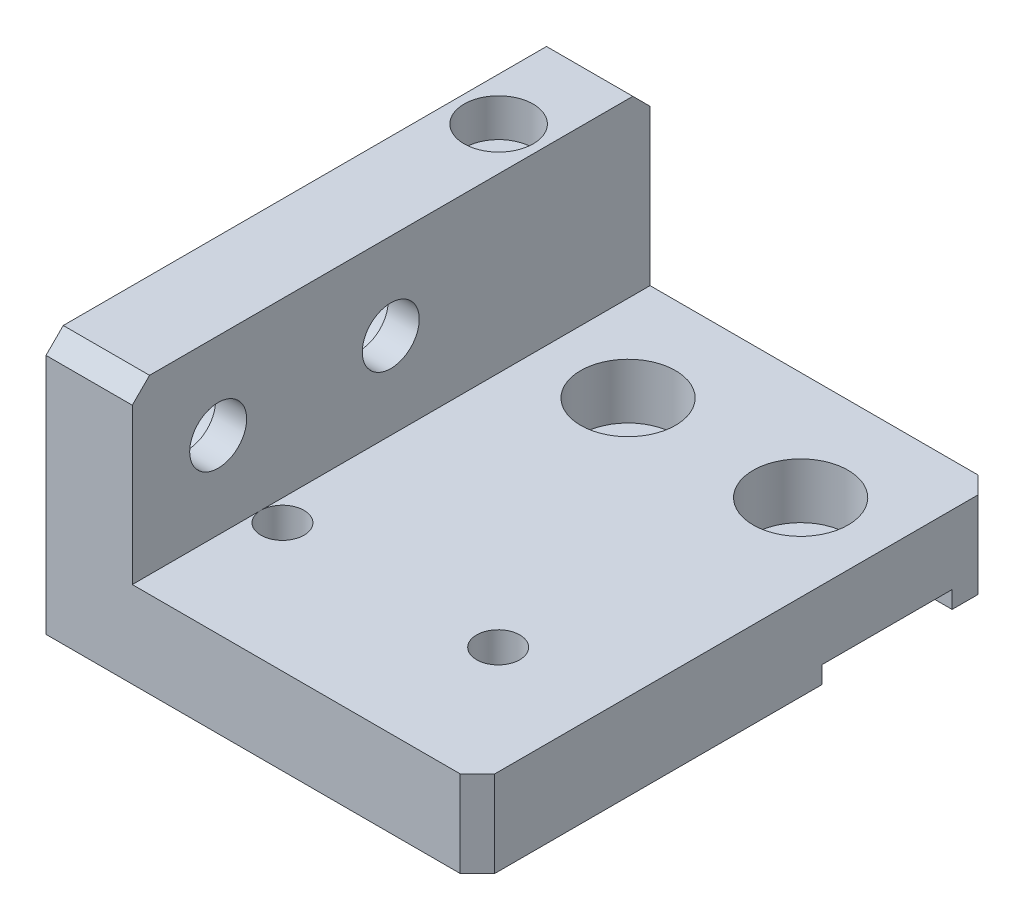
SolidWorks part; units mm, degrees
material "6061-T6"
ref_plane "前视基准面" through (0, 0, 0) normal (0, 0, 1) x (1, 0, 0)
ref_plane "上视基准面" through (0, 0, 0) normal (0, 1, 0) x (1, 0, 0)
ref_plane "右视基准面" through (0, 0, 0) normal (1, 0, 0) x (0, 0, -1)
sketch "草图2" plane through (0, 0, 0) normal (0, 0, 1) x (1, 0, 0)
  line L0 (50, 0) -> (0, 0)
  line L1 (0, 0) -> (0, 30)
  line L2 (50, 10) -> (10, 10)
  line L3 (10, 10) -> (10, 30)
  line L4 (10, 30) -> (0, 30)
  line L5 (50, 10) -> (50, 0)
  dimension "D1" = 50
  dimension "D2" = 30
  dimension "D3" = 10
extrude "凸台-拉伸1" add sketch "草图2" along normal blind 60
sketch "草图3" plane through (0, 0, 0) normal (0, -1, 0) x (1, 0, 0)
  line L0 (0, 60) -> (0, 0) construction
  line L1 (0, 20.1) -> (50, 20.1)
  line L2 (0, 20.1) -> (0, 5)
  line L3 (0, 5) -> (50, 5)
  line L4 (50, 20.1) -> (50, 5)
  line L5 (50, 60) -> (50, 0) construction
  line L7 (0, 0) -> (50, 0) construction
  dimension "D1" = 15.1
  dimension "D2" = 5
extrude "切除-拉伸1" cut sketch "草图3" against normal blind 2
hole_wizard "M4 六角凹头螺钉的柱形沉头孔1" positions "草图6" profile "草图5" counterbore size "M4" standard "ISO" end condition through all
sketch "草图6" plane through (0, 30, 0) normal (0, 1, 0) x (1, 0, 0)
  line L1 (25, -5) -> (25, -20.1) construction
  line L2 (0, -5) -> (50, -5) construction
  line L3 (50, -20.1) -> (0, -20.1) construction
  line L5 (25, -12.55) -> (5, -12.55) construction
  line L7 (5, -12.55) -> (5, 0) construction
  line L8 (10, 0) -> (0, 0) construction
  point P0 (5, -12.55)
sketch "草图5" plane through (5, 30, 12.55) normal (1, 0, 0) x (0, 0, 1)
  line L0 (0, 0) -> (0, 30)
  line L1 (0, 30) -> (2.25, 30)
  line L3 (2.25, 30) -> (2.25, 4.4)
  line L4 (2.25, 4.4) -> (4, 4.4)
  line L5 (4, 4.4) -> (4, 0)
  line L7 (4, 0) -> (0, 0)
  line L11 (0, -6.35) -> (0, 107.95) construction
  dimension "通孔孔直径" = 4.5
  dimension "通孔孔深度" = 30
  dimension "柱形沉头孔直径" = 8
  dimension "柱形沉头孔深度" = 4.4
hole_wizard "M6 六角凹头螺钉的柱形沉头孔1" positions "草图7" profile "草图8" counterbore size "M6" standard "ISO" end condition through all
sketch "草图7" plane through (0, 10, 0) normal (0, 1, 0) x (1, 0, 0)
  line L0 (40, -12.55) -> (20, -12.55) construction
  line L1 (20, -12.55) -> (5, -12.55) construction
  line L3 (30, -12.55) -> (30, 0) construction
  line L4 (50, 0) -> (10, 0) construction
  point P0 (20, -12.55)
  point P2 (40, -12.55)
  dimension "D1" = 20
sketch "草图8" plane through (20, 10, 12.55) normal (1, 0, 0) x (0, 0, 1)
  line L0 (0, 0) -> (0, 10)
  line L1 (0, 10) -> (3.3, 10)
  line L3 (3.3, 10) -> (3.3, 6.4)
  line L4 (3.3, 6.4) -> (5.5, 6.4)
  line L5 (5.5, 6.4) -> (5.5, 0)
  line L7 (5.5, 0) -> (0, 0)
  line L11 (0, -6.35) -> (0, 107.95) construction
  dimension "通孔孔直径" = 6.6
  dimension "通孔孔深度" = 10
  dimension "柱形沉头孔直径" = 11
  dimension "柱形沉头孔深度" = 6.4
hole_wizard "M6 六角凹头螺钉的柱形沉头孔2" positions "草图9" profile "草图10" counterbore size "M6" standard "ISO" end condition through all
sketch "草图9" plane through (0, 0, 0) normal (-1, 0, 0) x (0, 0, 1)
  line L0 (20.1, 0) -> (20.1, 30) construction
  line L1 (60, 30) -> (0, 30) construction
  line L3 (20.1, 20) -> (30.05, 20) construction
  line L4 (30.05, 20) -> (50.05, 20) construction
  line L6 (40.05, 20) -> (40.05, 0) construction
  line L7 (60, 0) -> (20.1, 0) construction
  point P0 (30.05, 20)
  point P2 (50.05, 20)
  dimension "D1" = 20
  dimension "D2" = 10
sketch "草图10" plane through (0, 20, 30.05) normal (0, 1, 0) x (0, 0, 1)
  line L0 (0, 0) -> (0, 50)
  line L1 (0, 50) -> (3.3, 50)
  line L3 (3.3, 50) -> (3.3, 6.4)
  line L4 (3.3, 6.4) -> (5.5, 6.4)
  line L5 (5.5, 6.4) -> (5.5, 0)
  line L7 (5.5, 0) -> (0, 0)
  line L11 (0, -6.35) -> (0, 107.95) construction
  dimension "通孔孔直径" = 6.6
  dimension "通孔孔深度" = 50
  dimension "柱形沉头孔直径" = 11
  dimension "柱形沉头孔深度" = 6.4
chamfer "倒角1" distance 2 angle 45 4 edges at (50, 5, 60) (50, 5, 0) (5, 30, 0) (5, 30, 60)
hole_wizard "M6 螺纹孔1" positions "草图11" profile "草图12" tap size "M6" standard "ISO"
sketch "草图11" plane through (0, 0, 0) normal (0, -1, 0) x (-1, 0, 0)
  point P0 (-37.5, -45.1)
  point P2 (-12.5, -45.1)
sketch "草图12" plane through (37.5, 0, 45.1) normal (1, 0, 0) x (0, 0, -1)
  line L0 (0, 0) -> (0, 18.5022)
  line L1 (0, 18.5022) -> (2.5, 17)
  line L2 (2.5, 17) -> (2.5, 0)
  line L5 (2.5, 0) -> (0, 0)
  line L10 (0, 18.5022) -> (-2.5, 17) construction
  line L11 (0, -6.35) -> (0, 107.95) construction
  dimension "螺纹孔钻头直径" = 5
  dimension "螺纹孔钻头深度" = 17
  dimension "导头角度" = 118
cosmetic thread "孔螺蚊线1" parameters "D1"=10, "D2"=6
cosmetic thread "孔螺蚊线2" parameters "D1"=10, "D2"=6
